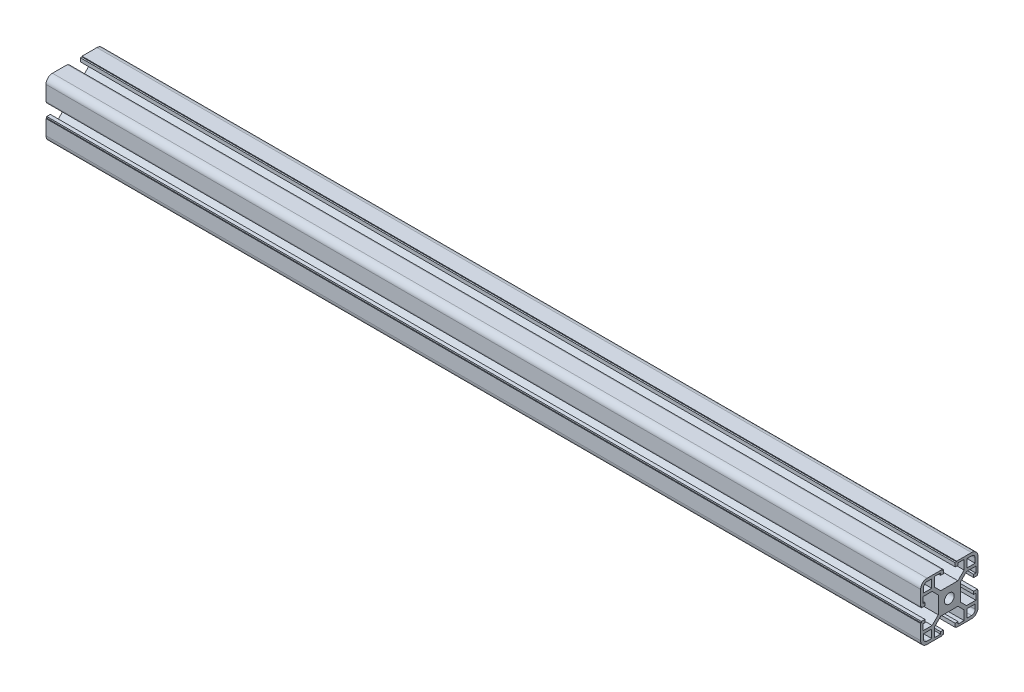
SolidWorks part; units mm, degrees
ref_plane "Front Plane" through (0, 0, 0) normal (0, 0, 1) x (1, 0, 0)
ref_plane "Top Plane" through (0, 0, 0) normal (0, 1, 0) x (1, 0, 0)
ref_plane "Right Plane" through (0, 0, 0) normal (1, 0, 0) x (0, 0, -1)
sketch "草图1" plane through (0, 0, 0) normal (0, 0, 1) x (1, 0, 0)
  line L0 (-984.975, 0) -> (-374.975, 0)
  dimension "D1" = 610
other "Aluminium profile 40 X 40B X R4.5(1)"
ref_plane "Plane1" through (-984.975, 0, 0) normal (1, 0, 0) x (0, 1, 0)
sketch "Sketch1" plane through (-984.975, 0, 0) normal (1, 0, 0) x (0, 1, 0)
  line L0 (-5.1, 20) -> (-5.1, 19.5)
  line L1 (-5.1, 19.5) -> (-4.1, 19.5)
  line L2 (-4.1, 19.5) -> (-4.1, 17)
  line L3 (-6.1, 18.5) -> (-10.3, 18.5)
  line L4 (-15.5, -20) -> (-5.1, -20)
  line L5 (-20, -15.5) -> (-20, -5.1)
  line L6 (15.5, 20) -> (5.1, 20)
  line L7 (20, 15.5) -> (20, 5.1)
  line L8 (0, 14.8756) -> (0, 0) construction
  line L9 (0, 0) -> (14.1675, 0) construction
  line L10 (-10.3, 18.5) -> (-10.3, 12)
  line L11 (-10.3, 12) -> (-6, 7.7)
  line L12 (-6, 7.7) -> (6, 7.7)
  line L13 (10.3, 12) -> (6, 7.7)
  line L14 (10.3, 18.5) -> (10.3, 12)
  line L15 (6.1, 18.5) -> (10.3, 18.5)
  line L16 (4.1, 19.5) -> (4.1, 17)
  line L17 (5.1, 19.5) -> (4.1, 19.5)
  line L18 (5.1, 20) -> (5.1, 19.5)
  line L19 (-5.1, 20) -> (-15.5, 20)
  line L20 (20, 5.1) -> (19.5, 5.1)
  line L21 (12.3, 18) -> (15.5, 18)
  line L22 (12.3, 18) -> (12.3, 12.3)
  line L23 (12.3, 12.3) -> (18, 12.3)
  line L24 (18, 15.5) -> (18, 12.3)
  line L25 (19.5, 5.1) -> (19.5, 4.1)
  line L26 (19.5, 4.1) -> (17, 4.1)
  line L27 (17, 6.1) -> (17, 4.1)
  line L28 (18.5, 6.1) -> (17, 6.1)
  line L29 (18.5, 6.1) -> (18.5, 10.3)
  line L30 (18.5, 10.3) -> (12, 10.3)
  line L31 (12, 10.3) -> (7.7, 6)
  line L32 (7.7, 6) -> (7.7, -6)
  line L33 (12, -10.3) -> (7.7, -6)
  line L34 (18.5, -10.3) -> (12, -10.3)
  line L35 (18.5, -6.1) -> (18.5, -10.3)
  line L36 (18.5, -6.1) -> (17, -6.1)
  line L37 (17, -4.1) -> (17, -6.1)
  line L38 (19.5, -4.1) -> (17, -4.1)
  line L39 (19.5, -5.1) -> (19.5, -4.1)
  line L40 (20, -5.1) -> (19.5, -5.1)
  line L41 (5.1, -20) -> (5.1, -19.5)
  line L42 (5.1, -19.5) -> (4.1, -19.5)
  line L43 (4.1, -19.5) -> (4.1, -17)
  line L44 (6.1, -17) -> (4.1, -17)
  line L45 (6.1, -18.5) -> (6.1, -17)
  line L46 (6.1, -18.5) -> (10.3, -18.5)
  line L47 (10.3, -18.5) -> (10.3, -12)
  line L48 (10.3, -12) -> (6, -7.7)
  line L49 (6, -7.7) -> (-6, -7.7)
  line L50 (-10.3, -12) -> (-6, -7.7)
  line L51 (-10.3, -18.5) -> (-10.3, -12)
  line L52 (-6.1, -18.5) -> (-10.3, -18.5)
  line L53 (-6.1, -18.5) -> (-6.1, -17)
  line L54 (-4.1, -17) -> (-6.1, -17)
  line L55 (-4.1, -19.5) -> (-4.1, -17)
  line L56 (-5.1, -19.5) -> (-4.1, -19.5)
  line L57 (-5.1, -20) -> (-5.1, -19.5)
  line L58 (-20, -5.1) -> (-19.5, -5.1)
  line L59 (5.1, -20) -> (15.5, -20)
  line L60 (-20, 5.1) -> (-20, 15.5)
  line L61 (-19.5, -5.1) -> (-19.5, -4.1)
  line L62 (-6.1, 18.5) -> (-6.1, 17)
  line L63 (-6.1, 17) -> (-4.1, 17)
  line L64 (6.1, 18.5) -> (6.1, 17)
  line L65 (4.1, 17) -> (6.1, 17)
  line L66 (-19.5, -4.1) -> (-17, -4.1)
  line L67 (-15.5, 18) -> (-12.3, 18)
  line L68 (-18, 15.5) -> (-18, 12.3)
  line L69 (-18, 12.3) -> (-12.3, 12.3)
  line L70 (-12.3, 18) -> (-12.3, 12.3)
  line L71 (-17, -6.1) -> (-17, -4.1)
  line L72 (-18.5, -6.1) -> (-17, -6.1)
  line L73 (-18.5, -6.1) -> (-18.5, -10.3)
  line L74 (-18.5, -10.3) -> (-12, -10.3)
  line L75 (-12, -10.3) -> (-7.7, -6)
  line L76 (-7.7, -6) -> (-7.7, 6)
  line L77 (-12, 10.3) -> (-7.7, 6)
  line L78 (-18.5, 10.3) -> (-12, 10.3)
  line L79 (-18.5, 6.1) -> (-18.5, 10.3)
  line L80 (-18.5, 6.1) -> (-17, 6.1)
  line L81 (-17, 4.1) -> (-17, 6.1)
  line L82 (-19.5, 4.1) -> (-17, 4.1)
  line L83 (-19.5, 5.1) -> (-19.5, 4.1)
  line L84 (-20, 5.1) -> (-19.5, 5.1)
  line L85 (20, -5.1) -> (20, -15.5)
  line L87 (-18, -12.3) -> (-12.3, -12.3)
  line L88 (-18, -12.3) -> (-18, -15.5)
  line L89 (-15.5, -18) -> (-12.3, -18)
  line L90 (-12.3, -12.3) -> (-12.3, -18)
  line L91 (12.3, -12.3) -> (18, -12.3)
  line L92 (12.3, -12.3) -> (12.3, -18)
  line L93 (12.3, -18) -> (15.5, -18)
  line L94 (18, -12.3) -> (18, -15.5)
  circle A0 centre (0, 0) radius 3.4
  arc A1 (-20, 15.5) -> (-15.5, 20) centre (-15.5, 15.5) cw
  arc A2 (20, 15.5) -> (15.5, 20) centre (15.5, 15.5) ccw
  arc A3 (-15.5, -20) -> (-20, -15.5) centre (-15.5, -15.5) cw
  arc A4 (15.5, -20) -> (20, -15.5) centre (15.5, -15.5) ccw
  arc A5 (-15.5, 18) -> (-18, 15.5) centre (-15.5, 15.5) ccw
  arc A6 (18, 15.5) -> (15.5, 18) centre (15.5, 15.5) ccw
  arc A7 (18, -15.5) -> (15.5, -18) centre (15.5, -15.5) cw
  arc A8 (-18, -15.5) -> (-15.5, -18) centre (-15.5, -15.5) ccw
  point P2 (0, 10)
  point P4 (0, 0)
  point P5 (-20, -20)
  point P6 (20, -20)
  point P7 (20, 20)
  point P8 (-20, 20)
  point P36 (-20, 20)
  point P39 (20, 20)
  point P121 (0, 0)
  dimension "D1" = 20.6
  dimension "D2" = 40
  dimension "D3" = 8.2
  dimension "D4" = 10.2
  dimension "D5" = 12.3
  dimension "D6" = 6.8
  dimension "D7" = 4.5
  dimension "D8" = 45
  dimension "D12" = 2
  dimension "D13" = 5.7
  dimension "D14" = 2
  dimension "D18" = 2.5
  dimension "D19" = 2.5
  dimension "D15" = 2.5
  dimension "D9" = 0.5
  dimension "D10" = 1.5
  dimension "D11" = 12
  dimension "D16" = 3
  dimension "D17" = 2
  dimension "D20" = 2
  dimension "D21" = 2
